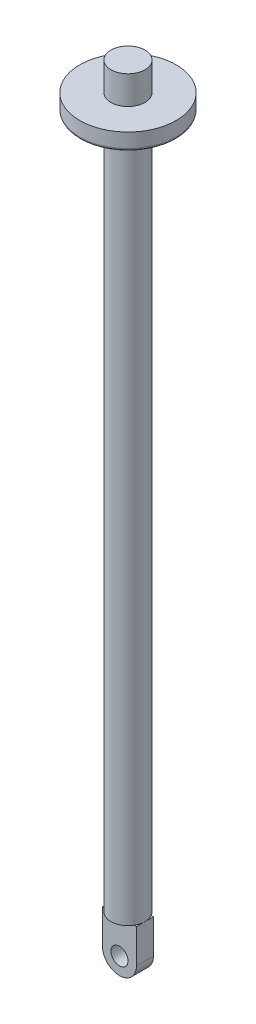
SolidWorks part; units mm, degrees
ref_plane "Front Plane" through (0, 0, 0) normal (0, 0, 1) x (1, 0, 0)
ref_plane "Top Plane" through (0, 0, 0) normal (0, 1, 0) x (1, 0, 0)
ref_plane "Right Plane" through (0, 0, 0) normal (1, 0, 0) x (0, 0, -1)
other "Configuration Table"
sketch "Sketch1" plane through (0, 0, 0) normal (0, 1, 0) x (1, 0, 0)
  circle A0 centre (0, 0) radius 3
  dimension "D1" = 6
extrude "Boss-Extrude1" add sketch "Sketch1" along normal blind 130
sketch "Sketch2" plane through (0, 0, 0) normal (0, 0, 1) x (1, 0, 0)
  line L0 (-3, 0) -> (-3, -6)
  line L1 (3, 0) -> (3, -6)
  line L2 (-3, 0) -> (3, 0)
  circle A0 centre (0, -6) radius 3
  circle A1 centre (0, -6) radius 1.5
  dimension "D1" = 3
  dimension "D2" = 6
extrude "Boss-Extrude2" add sketch "Sketch2" along normal mid plane 3 contours A0 L1 L2 L0 | A0 A1
ref_plane "Plane1" through (0, 122, 0) normal (0, 1, 0) x (1, 0, 0)
sketch "Sketch3" plane through (0, 122, 0) normal (0, 1, 0) x (1, 0, 0)
  circle A0 centre (0, 0) radius 8.5
  dimension "D1" = 17
extrude "Boss-Extrude3" add sketch "Sketch3" along normal blind 3
fillet "Fillet1" radius 0.5 1 edges at (0, 122, 8.5)
